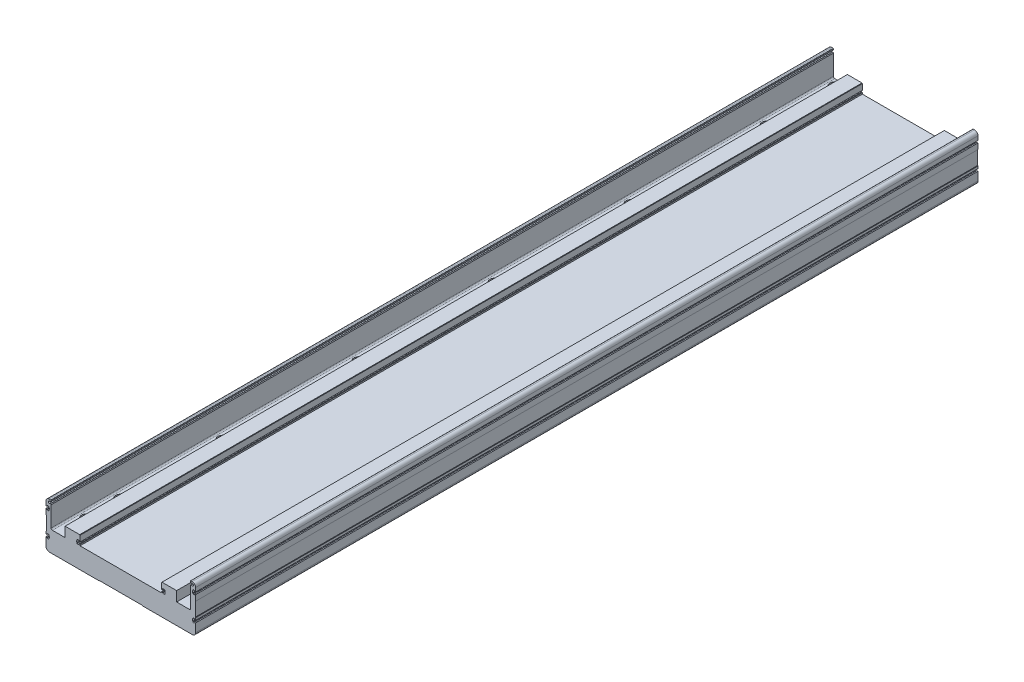
SolidWorks part; units mm, degrees
material "6063-T5"
ref_plane "前视基准面" through (0, 0, 0) normal (0, 0, 1) x (1, 0, 0)
ref_plane "上视基准面" through (0, 0, 0) normal (0, 1, 0) x (1, 0, 0)
ref_plane "右视基准面" through (0, 0, 0) normal (1, 0, 0) x (0, 0, -1)
sketch "草图1" plane through (0, 0, 0) normal (0, 0, 1) x (1, 0, 0)
  line L0 (0, -1000) -> (0, 49000) construction
  line L1 (-1000, 0) -> (-105, 0) construction
  line L2 (-104, 0) -> (-33.5, 0)
  line L3 (-33.5, 0) -> (-32, 1.5)
  line L4 (-32, 1.5) -> (32, 1.5)
  line L6 (-103.3917, 65.5661) -> (-102.5, 66.4578)
  line L7 (105, 64.5) -> (102.5, 64.5) construction
  line L8 (-103.3917, 63.4339) -> (-102.5, 62.5422)
  line L9 (110, 6) -> (110, 18.35)
  line L10 (105, 1) -> (104, 0)
  line L11 (-60, 31.5) -> (60, 31.5)
  line L12 (-110, 46) -> (-109.5, 45.5)
  line L15 (103.3917, 63.4339) -> (102.5, 62.5422)
  line L16 (-105, 64.5) -> (-102.5, 64.5) construction
  line L17 (82, 31) -> (102.5, 31)
  line L18 (103.3917, 65.5661) -> (102.5, 66.4578)
  line L19 (-102.5, 66.4578) -> (-102.5, 68)
  line L20 (105, 68.5) -> (103, 68.5)
  line L21 (-105, 68.5) -> (-103, 68.5)
  line L22 (102.5, 66.4578) -> (102.5, 68)
  line L24 (-82, 31) -> (-102.5, 31)
  line L25 (-105, 1) -> (-104, 0)
  line L26 (-104, 0) -> (104, 0) construction
  line L27 (-62.9, 34.9) -> (-62.9, 37.8) construction
  line L29 (-60, 33.5) -> (-60, 31.5)
  line L30 (-62, 47) -> (-60, 45)
  line L31 (-110, 6) -> (-110, 18.35)
  line L32 (-82, 31) -> (-82, 47)
  line L33 (-82, 47) -> (-62, 47)
  line L35 (62, 47) -> (60, 45)
  line L36 (33.5, 0) -> (32, 1.5)
  line L37 (33.5, 0) -> (104, 0)
  line L39 (-61.2, 33.5) -> (-61.2, 32)
  line L41 (102.5, 31) -> (102.5, 62.5422)
  line L42 (-102.5, 31) -> (-102.5, 62.5422)
  line L43 (-110, 21.65) -> (-110, 25)
  line L44 (62, 47) -> (82, 47)
  line L45 (82, 31) -> (82, 47)
  line L46 (-60.2, 33.7) -> (-61, 33.7)
  line L47 (-61.2, 37.8) -> (-64.6, 37.8)
  line L48 (-61.2, 37.8) -> (-61.2, 36.3)
  line L49 (-61.2, 32) -> (-64.6, 32)
  line L50 (-64.6, 37.8) -> (-64.6, 36.1329)
  line L51 (-61.2, 37.8) -> (-64.6, 32) construction
  line L52 (-107.1, 20) -> (-107.1, 22.9) construction
  line L53 (-108.4, 18.35) -> (-108.4, 17.1)
  line L54 (-110, 18.35) -> (-108.4, 18.35)
  line L55 (-108.4, 22.9) -> (-105.8, 22.9)
  line L56 (-108.4, 22.9) -> (-108.4, 21.65)
  line L57 (-108.4, 17.1) -> (-105.8, 17.1)
  line L58 (-105.8, 22.9) -> (-105.8, 21.6492)
  line L59 (-108.4, 22.9) -> (-105.8, 17.1) construction
  line L60 (-108.4, 17.1) -> (-105.8, 22.9) construction
  line L61 (-105.8, 18.3508) -> (-105.8, 17.1)
  line L62 (-108.4, 21.65) -> (-110, 21.65)
  line L63 (-107.1, 20) -> (-102.8, 20) construction
  line L65 (-61.2, 32) -> (-64.6, 37.8) construction
  line L68 (-107.1, 56) -> (-107.1, 58.9) construction
  line L69 (-108.4, 54.35) -> (-108.4, 53.1)
  line L70 (-110, 54.35) -> (-108.4, 54.35)
  line L71 (-108.4, 58.9) -> (-105.8, 58.9)
  line L72 (-108.4, 58.9) -> (-108.4, 57.65)
  line L73 (-108.4, 53.1) -> (-105.8, 53.1)
  line L74 (-105.8, 58.9) -> (-105.8, 57.6492)
  line L75 (-108.4, 58.9) -> (-105.8, 53.1) construction
  line L76 (-108.4, 53.1) -> (-105.8, 58.9) construction
  line L77 (-105.8, 54.3508) -> (-105.8, 53.1)
  line L78 (-108.4, 57.65) -> (-110, 57.65)
  line L79 (-107.1, 56) -> (-105, 56) construction
  line L80 (-110, 57.65) -> (-110, 63.5)
  line L81 (-64.6, 33.6671) -> (-64.6, 32)
  line L82 (108.4, 17.1) -> (105.8, 22.9) construction
  line L83 (108.4, 22.9) -> (105.8, 17.1) construction
  line L84 (107.1, 20) -> (107.1, 22.9) construction
  line L85 (108.4, 21.65) -> (110, 21.65)
  line L86 (105.8, 18.3508) -> (105.8, 17.1)
  line L87 (105.8, 22.9) -> (105.8, 21.6492)
  line L88 (108.4, 17.1) -> (105.8, 17.1)
  line L89 (108.4, 22.9) -> (108.4, 21.65)
  line L90 (108.4, 22.9) -> (105.8, 22.9)
  line L91 (110, 18.35) -> (108.4, 18.35)
  line L92 (108.4, 18.35) -> (108.4, 17.1)
  line L93 (107.1, 56) -> (105, 56) construction
  line L94 (108.4, 53.1) -> (105.8, 58.9) construction
  line L95 (108.4, 58.9) -> (105.8, 53.1) construction
  line L96 (107.1, 56) -> (107.1, 58.9) construction
  line L97 (108.4, 57.65) -> (110, 57.65)
  line L98 (105.8, 54.3508) -> (105.8, 53.1)
  line L99 (105.8, 58.9) -> (105.8, 57.6492)
  line L100 (108.4, 53.1) -> (105.8, 53.1)
  line L101 (108.4, 58.9) -> (108.4, 57.65)
  line L102 (108.4, 58.9) -> (105.8, 58.9)
  line L103 (110, 54.35) -> (108.4, 54.35)
  line L104 (108.4, 54.35) -> (108.4, 53.1)
  line L105 (110, 57.65) -> (110, 63.5)
  line L106 (110, 21.65) -> (110, 25)
  line L107 (-61, 36.1) -> (-60.2, 36.1)
  line L108 (-62.9, 34.9) -> (-45.8657, 34.9) construction
  line L109 (62.9, 34.9) -> (45.8657, 34.9) construction
  line L110 (61.2, 32) -> (64.6, 37.8) construction
  line L111 (61.2, 37.8) -> (64.6, 32) construction
  line L112 (62.9, 34.9) -> (62.9, 37.8) construction
  line L113 (61, 36.1) -> (60.2, 36.1)
  line L114 (64.6, 33.6671) -> (64.6, 32)
  line L115 (64.6, 37.8) -> (64.6, 36.1329)
  line L116 (61.2, 32) -> (64.6, 32)
  line L117 (61.2, 37.8) -> (61.2, 36.3)
  line L118 (61.2, 37.8) -> (64.6, 37.8)
  line L119 (60.2, 33.7) -> (61, 33.7)
  line L120 (61.2, 33.5) -> (61.2, 32)
  line L121 (60, 45) -> (60, 36.3)
  line L124 (60, 33.5) -> (60, 31.5)
  line L128 (-109.5, 45.5) -> (-109.5, 25.5)
  line L132 (-109.5, 25.5) -> (-110, 25)
  line L133 (-109.5, 35.5) -> (-42.499, 35.5) construction
  line L134 (-110, 46) -> (-110, 54.35)
  line L135 (109.5, 35.5) -> (42.499, 35.5) construction
  line L136 (109.5, 25.5) -> (110, 25)
  line L137 (109.5, 45.5) -> (109.5, 25.5)
  line L138 (110, 46) -> (109.5, 45.5)
  line L139 (110, 46) -> (110, 54.35)
  line L158 (-60, 45) -> (-60, 36.3)
  arc A0 (-103.6875, 65.5804) -> (-103.6875, 63.4196) centre (-105, 64.5) ccw
  arc A1 (103.3917, 63.4339) -> (103.6875, 63.4196) centre (103.5331, 63.2925) cw
  arc A2 (-110, 6) -> (-105, 1) centre (-105, 6) ccw
  arc A3 (105, 1) -> (110, 6) centre (105, 6) ccw
  arc A4 (-105.8, 54.3508) -> (-105.8, 57.6492) centre (-107.1, 56) ccw
  arc A5 (-103.3917, 65.5661) -> (-103.6875, 65.5804) centre (-103.5331, 65.7075) cw
  arc A6 (-103.3917, 63.4339) -> (-103.6875, 63.4196) centre (-103.5331, 63.2925) ccw
  arc A7 (103.3917, 65.5661) -> (103.6875, 65.5804) centre (103.5331, 65.7075) ccw
  arc A8 (-105, 68.5) -> (-110, 63.5) centre (-105, 63.5) ccw
  arc A9 (110, 63.5) -> (105, 68.5) centre (105, 63.5) ccw
  arc A10 (103.6875, 65.5804) -> (103.6875, 63.4196) centre (105, 64.5) cw
  arc A11 (102.5, 68) -> (103, 68.5) centre (103, 68) cw
  arc A12 (-102.5, 68) -> (-103, 68.5) centre (-103, 68) ccw
  arc A13 (-64.6, 36.1329) -> (-64.6, 33.6671) centre (-62.9, 34.9) ccw
  arc A15 (60.2, 33.7) -> (60, 33.5) centre (60.2, 33.5) ccw
  arc A16 (-105.8, 18.3508) -> (-105.8, 21.6492) centre (-107.1, 20) ccw
  arc A17 (64.6, 36.1329) -> (64.6, 33.6671) centre (62.9, 34.9) cw
  arc A18 (105.8, 18.3508) -> (105.8, 21.6492) centre (107.1, 20) cw
  arc A19 (105.8, 54.3508) -> (105.8, 57.6492) centre (107.1, 56) cw
  arc A27 (61, 33.7) -> (61.2, 33.5) centre (61, 33.5) cw
  arc A41 (61, 36.1) -> (61.2, 36.3) centre (61, 36.3) ccw
  arc A42 (60.2, 36.1) -> (60, 36.3) centre (60.2, 36.3) cw
  arc A43 (-61.2, 33.5) -> (-61, 33.7) centre (-61, 33.5) cw
  arc A44 (-60.2, 33.7) -> (-60, 33.5) centre (-60.2, 33.5) cw
  arc A45 (-60, 36.3) -> (-60.2, 36.1) centre (-60.2, 36.3) cw
  arc A46 (-61, 36.1) -> (-61.2, 36.3) centre (-61, 36.3) cw
  point P35 (-60, 47)
  point P46 (-103.5578, 65.4)
  point P65 (-103.5578, 63.6)
  point P72 (103.5578, 63.6)
  point P73 (103.5578, 65.4)
  point P154 (60, 47)
  point P163 (60, 33.7)
  point P236 (102.8, 26)
  point P241 (61.2, 33.7)
  point P244 (61.2, 36.1)
  point P247 (60, 36.1)
  point P250 (-61.2, 33.7)
  point P253 (-60, 33.7)
  point P256 (-60, 36.1)
  point P259 (-61.2, 36.1)
  dimension "D18" = 2.5
  dimension "D22" = 0.5
  dimension "D4" = 210
  dimension "D16" = 90
  dimension "D20" = 1.8
  dimension "D24" = 1.6
  dimension "D27" = 2.1
  dimension "D17" = 4
  dimension "D15" = 3.4
  dimension "D6" = 10
  dimension "D19" = 1.5
  dimension "D28" = 10
  dimension "D37" = 3.4
  dimension "D38" = 2.4
  dimension "D39" = 20
  dimension "D40" = 0.2
  dimension "D47" = 3.3
  dimension "D51" = 2.1
  dimension "D25" = 0.2
  dimension "D65" = 22
  dimension "D3" = 7.5
  dimension "D5" = 220
  dimension "D7" = 68.5
  dimension "D8" = 1
  dimension "D9" = 64
  dimension "D10" = 30
  dimension "D12" = 82
  dimension "D21" = 31
  dimension "D26" = 45
  dimension "D31" = 45
  dimension "D32" = 45
  dimension "D33" = 1
  dimension "D34" = 1.2
  dimension "D35" = 3.4
  dimension "D43" = 3.3
  dimension "D44" = 2.6
  dimension "D45" = 5.8
  dimension "D49" = 2.6
  dimension "D50" = 5.8
  dimension "D52" = 1.6
  dimension "D53" = 56
  dimension "D36" = 5.8
  dimension "D61" = 45
  dimension "D62" = 0.5
  dimension "D63" = 20
  dimension "D64" = 35.5
extrude "凸台-拉伸1" add sketch "草图1" along normal mid plane 1150
fillet "圆角11" radius 2 2 edges at (102.5, 31, 0) (-102.5, 31, 0)
sketch "草图24" plane through (0, 0, 575) normal (0, 0, 1) x (1, 0, 0)
  line L0 (0, 0) -> (0, 39.3203) construction
  line L1 (110, 6) -> (110, 18.35) construction
  line L2 (-110, 0) -> (110, 0)
  line L3 (-110, 0) -> (-110, 1)
  line L4 (-110, 1) -> (110, 1)
  line L5 (110, 0) -> (110, 1)
  line L6 (-110, 18.35) -> (-110, 6) construction
  line L8 (-104, 0) -> (-33.5, 0) construction
  dimension "D1" = 1
extrude "切除-拉伸8" cut sketch "草图24" against normal through all
sketch "草图6" plane through (0, 0, -575) normal (0, 0, -1) x (-1, 0, 0)
  line L1 (-53, 45.5) -> (-83, 45.5)
  line L2 (-53, 45.5) -> (-53, 50.5)
  line L3 (-53, 50.5) -> (-83, 50.5)
  line L4 (-83, 45.5) -> (-83, 50.5)
  line L5 (-82, 47) -> (-62, 47) construction
  line L6 (53, 45.5) -> (83, 45.5)
  line L7 (53, 45.5) -> (53, 50.5)
  line L8 (53, 50.5) -> (83, 50.5)
  line L9 (83, 45.5) -> (83, 50.5)
  line L11 (0, 0) -> (0, 47.4202) construction
  dimension "D1" = 1.5
  dimension "D2" = 166
  dimension "D3" = 5
  dimension "D4" = 30
extrude "切除-拉伸5" cut sketch "草图6" against normal through all
hole_wizard "打孔尺寸根据内六角圆柱头螺钉的类型4" positions "草图17" profile "草图16" counterbore size "M8" standard "GB" end condition through all
sketch "草图17" plane through (268.5044, 31, 525.7239) normal (0, 1, 0) x (1, 0, 0)
  line L0 (-268.5044, 1100.7239) -> (-268.5044, -49.2761) construction
  line L1 (-208.5044, 1100.7239) -> (-328.5044, 1100.7239) construction
  line L2 (-350.5044, 1100.7239) -> (-369.0044, 1100.7239) construction
  line L3 (-208.5044, -49.2761) -> (-328.5044, -49.2761) construction
  point P0 (-359.5044, 991.7239)
  point P2 (-177.5044, 991.7239)
  point P13 (-359.7544, 1100.7239)
  dimension "D1" = 182
  dimension "D2" = 109
sketch "草图16" plane through (-91, 31, -466) normal (1, 0, 0) x (0, 0, 1)
  line L0 (0, 0) -> (0, 30)
  line L1 (0, 30) -> (4.3, 30)
  line L3 (4.3, 30) -> (4.3, 18)
  line L4 (4.3, 18) -> (7.5, 18)
  line L5 (7.5, 18) -> (7.5, 0)
  line L7 (7.5, 0) -> (0, 0)
  line L11 (0, -6.35) -> (0, 107.95) construction
  dimension "通孔孔直径" = 8.6
  dimension "通孔孔深度" = 30
  dimension "柱形沉头孔直径" = 15
  dimension "柱形沉头孔深度" = 18
cosmetic thread "装饰螺纹线9" parameters "D2"=10
cosmetic thread "装饰螺纹线10" parameters "D2"=10
hole_wizard "打孔尺寸根据内六角圆柱头螺钉的类型4" positions "草图19" profile "草图18" counterbore size "M8" standard "GB" end condition through all
sketch "草图19" plane through (-106.5882, 31, 143.2622) normal (0, 1, 0) x (1, 0, 0)
  line L0 (106.5882, -431.7378) -> (106.5882, -43.6262) construction
  line L1 (166.5882, -431.7378) -> (46.5882, -431.7378) construction
  line L3 (207.0882, -431.7378) -> (188.5882, -431.7378) construction
  point P0 (197.5882, -340.7378)
  point P2 (15.5882, -340.7378)
  dimension "D2" = 182
  dimension "D1" = 91
sketch "草图18" plane through (91, 31, 484) normal (1, 0, 0) x (0, 0, 1)
  line L0 (0, 0) -> (0, 30)
  line L1 (0, 30) -> (4.3, 30)
  line L3 (4.3, 30) -> (4.3, 18)
  line L4 (4.3, 18) -> (7.5, 18)
  line L5 (7.5, 18) -> (7.5, 0)
  line L7 (7.5, 0) -> (0, 0)
  line L11 (0, -6.35) -> (0, 107.95) construction
  dimension "通孔孔直径" = 8.6
  dimension "通孔孔深度" = 30
  dimension "柱形沉头孔直径" = 15
  dimension "柱形沉头孔深度" = 18
cosmetic thread "装饰螺纹线2" parameters "D2"=10
cosmetic thread "装饰螺纹线3" parameters "D2"=10
pattern_linear "阵列(线性)2" count 5 spacing 200 along (0, 0, 1) of "打孔尺寸根据内六角圆柱头螺钉的类型4"
hole_wizard "打孔尺寸根据内六角圆柱头螺钉的类型4" positions "草图45" profile "草图44" counterbore size "M8" standard "GB" end condition through all
sketch "草图45" plane through (87.9576, 31, 219.2964) normal (0, 1, 0) x (1, 0, 0)
  line L0 (3.0424, -264.7036) -> (3.0424, 785.2964) construction
  line L2 (-178.9576, -264.7036) -> (-178.9576, 785.2964) construction
  line L3 (3.0424, -264.7036) -> (3.0424, -314.7036) construction
  line L5 (-178.9576, -264.7036) -> (-178.9576, -314.7036) construction
  line L7 (12.5424, 794.2964) -> (-5.9576, 794.2964) construction
  line L8 (12.5424, -355.7036) -> (-5.9576, -355.7036) construction
  point P0 (3.0424, 785.2964)
  point P2 (-178.9576, 785.2964)
  point P14 (-178.9576, -314.7036)
  point P16 (3.0424, -314.7036)
  dimension "D1" = 9
  dimension "D2" = 41
sketch "草图44" plane through (91, 31, -566) normal (1, 0, 0) x (0, 0, 1)
  line L0 (0, 0) -> (0, 30)
  line L1 (0, 30) -> (4.3, 30)
  line L3 (4.3, 30) -> (4.3, 18)
  line L4 (4.3, 18) -> (7.5, 18)
  line L5 (7.5, 18) -> (7.5, 0)
  line L7 (7.5, 0) -> (0, 0)
  line L11 (0, -6.35) -> (0, 107.95) construction
  dimension "通孔孔直径" = 8.6
  dimension "通孔孔深度" = 30
  dimension "柱形沉头孔直径" = 15
  dimension "柱形沉头孔深度" = 18
cosmetic thread "装饰螺纹线1" parameters "D2"=10
cosmetic thread "装饰螺纹线4" parameters "D2"=10
cosmetic thread "装饰螺纹线7" parameters "D2"=10
cosmetic thread "装饰螺纹线8" parameters "D2"=10
sketch "草图46" plane through (0, 1.5, 0) normal (0, -1, 0) x (1, 0, 0)
  line L0 (0, -575) -> (0, 575) construction
  line L1 (-32, -575) -> (32, -575) construction
  line L2 (-32, 575) -> (32, 575) construction
  line L3 (-91, -566) -> (91, -566) construction
  line L4 (-91, 534) -> (91, 534) construction
  line L5 (0, -515) -> (0, -517) construction
  line L6 (3, -515) -> (3, -517)
  line L7 (-3, -515) -> (-3, -517)
  line L8 (0, 533) -> (0, 535) construction
  line L9 (-3, 533) -> (-3, 535)
  line L10 (3, 533) -> (3, 535)
  circle A0 centre (0, -566) radius 3
  arc A1 (3, -515) -> (-3, -515) centre (0, -515) ccw
  arc A2 (-3, -517) -> (3, -517) centre (0, -517) ccw
  arc A3 (-3, 533) -> (3, 533) centre (0, 533) ccw
  arc A4 (3, 535) -> (-3, 535) centre (0, 535) ccw
  circle A5 centre (0, 484) radius 3
  point P18 (0, -516)
  point P25 (0, 534)
  dimension "D1" = 6
  dimension "D2" = 2
  dimension "D4" = 2
  dimension "D5" = 3
  dimension "D3" = 50
  dimension "50" = 50
extrude "切除-拉伸9" cut sketch "草图46" against normal blind 8
